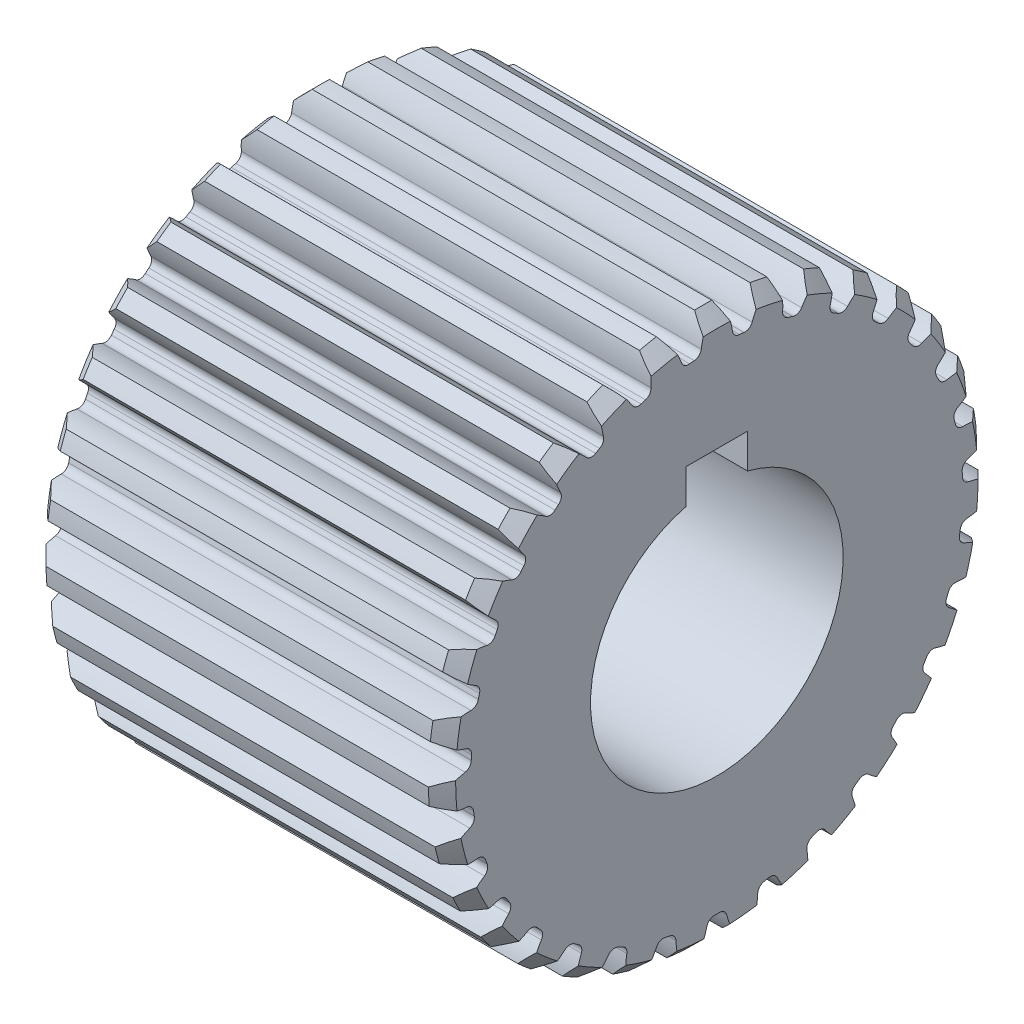
from build123d import *

# Parameters (mm, degrees)
SKETCH4_OUTSIDE_W   = 108.238
SKETCH4_OUTSIDE_H   = 108.238
CUT_EXTRUDE6_DEPTH  = 60
CUT_EXTRUDE7_REACH  = 84.701
SKETCH5_W           = 9
SKETCH5_H           = 23
BOSS_EXTRUDE1_DEPTH = 60
SCALE_1_SCALE       = 1.875


with BuildPart() as part:
    # Sketch1 → Revolve1 (revolve)
    with BuildSketch(Plane.XY, mode=Mode.PRIVATE) as revolve1_sk:
        Polygon((31.149526316, 18.25), (31.149526316, 38.25), (29.149526316, 40.25), (-26.850473684, 40.25), (-28.850473684, 38.25), (-28.850473684, 18.25), (-28.850473684, 0), (31.149526316, 0), align=None)
    revolve(revolve1_sk.sketch.rotate(Axis((-28.850473684, 0, 0), (1, 0, 0)), 90), axis=Axis((-28.850473684, 0, 0), (1, 0, 0)))

    # Sketch2 → Cut-Revolve1 (revolve, cut)
    with BuildSketch(Plane.XY, mode=Mode.PRIVATE) as cut_revolve1_sk:
        Polygon((0, 0), (44.149457516, 0), (44.149457516, 19), (-36.76595356, 19), (-36.76595356, 0), align=None)
    revolve(cut_revolve1_sk.sketch.rotate(Axis((-36.76595356, 0, 0), (1, 0, 0)), 90), axis=Axis((-36.76595356, 0, 0), (1, 0, 0)), mode=Mode.SUBTRACT)

    # Sketch4 outside → Cut-Extrude6 (cut)
    with BuildSketch(Plane.ZY.offset(28.850473684)):
        Rectangle(SKETCH4_OUTSIDE_W, SKETCH4_OUTSIDE_H)
        with BuildLine():
            ThreePointArc((1.260367328, 40.230261921), (0, 40.25), (-1.260367328, 40.230261921))
            ThreePointArc((-1.260367328, 40.230261921), (-1.890771319, 38.543683265), (-2.279945836, 36.785701483))
            ThreePointArc((-2.279945836, 36.785701483), (-2.625906951, 36.135179583), (-3.304440864, 35.84802185))
            ThreePointArc((-3.304440864, 35.84802185), (-3.642059592, 35.815295642), (-3.979354981, 35.779389793))
            ThreePointArc((-3.979354981, 35.779389793), (-4.701803692, 35.924081517), (-5.171632058, 36.491645735))
            ThreePointArc((-5.171632058, 36.491645735), (-5.906719281, 38.135301273), (-6.863724652, 39.660456174))
            ThreePointArc((-6.863724652, 39.660456174), (-8.102265434, 39.426080135), (-9.332859723, 39.153036018))
            ThreePointArc((-9.332859723, 39.153036018), (-9.61085352, 37.374082336), (-9.63818248, 35.573746289))
            ThreePointArc((-9.63818248, 35.573746289), (-9.846112655, 34.866899151), (-10.452952512, 34.449031681))
            ThreePointArc((-10.452952512, 34.449031681), (-10.777072427, 34.34901323), (-11.100235566, 34.245945313))
            ThreePointArc((-11.100235566, 34.245945313), (-11.837021939, 34.242247333), (-12.411482728, 34.703617723))
            ThreePointArc((-12.411482728, 34.703617723), (-13.462388099, 36.165655566), (-14.706814939, 37.466946691))
            ThreePointArc((-14.706814939, 37.466946691), (-15.872823168, 36.988051918), (-17.023263743, 36.47288022))
            ThreePointArc((-17.023263743, 36.47288022), (-16.937466247, 34.674382085), (-16.601830801, 32.905397744))
            ThreePointArc((-16.601830801, 32.905397744), (-16.663217349, 32.171163771), (-17.173519056, 31.639694108))
            ThreePointArc((-17.173519056, 31.639694108), (-17.470870651, 31.476478181), (-17.766671202, 31.310467809))
            ThreePointArc((-17.766671202, 31.310467809), (-18.487631117, 31.15853152), (-19.143205837, 31.494819525))
            ThreePointArc((-19.143205837, 31.494819525), (-20.466905167, 32.71538367), (-21.947806495, 33.739536009))
            ThreePointArc((-21.947806495, 33.739536009), (-22.993545658, 33.035728509), (-24.016733346, 32.299520421))
            ThreePointArc((-24.016733346, 32.299520421), (-23.570657117, 30.555108557), (-22.885798217, 28.889898348))
            ThreePointArc((-22.885798217, 28.889898348), (-22.798127968, 28.158337166), (-23.190999712, 27.53502374))
            ThreePointArc((-23.190999712, 27.53502374), (-23.449409378, 27.315292417), (-23.705737232, 27.093136073))
            ThreePointArc((-23.705737232, 27.093136073), (-24.381354505, 26.799181766), (-25.091203849, 26.996619714))
            ThreePointArc((-25.091203849, 26.996619714), (-26.633504733, 27.925740124), (-28.290252273, 28.630824758))
            ThreePointArc((-28.290252273, 28.630824758), (-29.172909686, 27.730918493), (-30.026955064, 26.80381446))
            ThreePointArc((-30.026955064, 26.80381446), (-29.238862515, 25.184905294), (-28.232818366, 23.691643119))
            ThreePointArc((-28.232818366, 23.691643119), (-27.999680549, 22.99270493), (-28.259038115, 22.303066265))
            ThreePointArc((-28.259038115, 22.303066265), (-28.46792653, 22.035815372), (-28.674287594, 21.766608164))
            ThreePointArc((-28.674287594, 21.766608164), (-29.276902375, 21.342670361), (-30.011965028, 21.39317512))
            ThreePointArc((-30.011965028, 21.39317512), (-31.709725486, 21.992813495), (-33.4744918, 22.349964178))
            ThreePointArc((-33.4744918, 22.349964178), (-34.157931364, 21.290801416), (-34.807869713, 20.210757186))
            ThreePointArc((-34.807869713, 20.210757186), (-33.710025446, 18.78362905), (-32.423983614, 17.523449238))
            ThreePointArc((-32.423983614, 17.523449238), (-32.054922918, 16.885748651), (-32.170148177, 16.158018637))
            ThreePointArc((-32.170148177, 16.158018637), (-32.320963425, 15.854189456), (-32.468909253, 15.548952759))
            ThreePointArc((-32.468909253, 15.548952759), (-32.973850422, 15.012387524), (-33.704032833, 14.913891424))
            ThreePointArc((-33.704032833, 14.913891424), (-35.487746352, 15.159498498), (-37.288281699, 15.154093438))
            ThreePointArc((-37.288281699, 15.154093438), (-37.744523319, 13.979036427), (-38.163746087, 12.790269139))
            ThreePointArc((-38.163746087, 12.790269139), (-36.801095974, 11.613348826), (-35.287707163, 10.637843285))
            ThreePointArc((-35.287707163, 10.637843285), (-34.797832977, 10.08748784), (-34.764208593, 9.351459827))
            ThreePointArc((-34.764208593, 9.351459827), (-34.850776279, 9.023491161), (-34.934249953, 8.694721401))
            ThreePointArc((-34.934249953, 8.694721401), (-35.320845158, 8.067495778), (-36.016253573, 7.82403126))
            ThreePointArc((-36.016253573, 7.82403126), (-37.812894712, 7.705551852), (-39.575484965, 7.337812332))
            ThreePointArc((-39.575484965, 7.337812332), (-39.785850054, 6.094968045), (-39.957194211, 4.84614597))
            ThreePointArc((-39.957194211, 4.84614597), (-38.385525309, 3.967616736), (-36.706747835, 3.316722779))
            ThreePointArc((-36.706747835, 3.316722779), (-36.116115665, 2.87624409), (-35.935018225, 2.162051153))
            ThreePointArc((-35.935018225, 2.162051153), (-35.953794258, 1.823370078), (-35.969378355, 1.484527127))
            ThreePointArc((-35.969378355, 1.484527127), (-36.221800344, 0.792319807), (-36.85396466, 0.413854337))
            ThreePointArc((-36.85396466, 0.413854337), (-38.58997872, -0.063860993), (-40.242463226, -0.778879672))
            ThreePointArc((-40.242463226, -0.778879672), (-40.198339414, -2.038629046), (-40.11479011, -3.296378984))
            ThreePointArc((-40.11479011, -3.296378984), (-38.398446728, -3.840550049), (-36.623009937, -4.140184747))
            ThreePointArc((-36.623009937, -4.140184747), (-35.955800335, -4.45275343), (-35.634643988, -5.115872149))
            ThreePointArc((-35.634643988, -5.115872149), (-35.584859676, -5.45139999), (-35.53191618, -5.786443862))
            ThreePointArc((-35.53191618, -5.786443862), (-35.639830767, -6.515293831), (-36.182870104, -7.013265831))
            ThreePointArc((-36.182870104, -7.013265831), (-37.787184465, -7.830659362), (-39.261910314, -8.863684252))
            ThreePointArc((-39.261910314, -8.863684252), (-38.965104034, -10.088764423), (-38.630081789, -11.303949796))
            ThreePointArc((-38.630081789, -11.303949796), (-36.839331227, -11.491484264), (-35.03992171, -11.427592624))
            ThreePointArc((-35.03992171, -11.427592624), (-34.323450314, -11.599454702), (-33.87538324, -12.184351044))
            ThreePointArc((-33.87538324, -12.184351044), (-33.759076757, -12.502989102), (-33.639773183, -12.820517159))
            ThreePointArc((-33.639773183, -12.820517159), (-33.598762332, -13.556170573), (-34.030444595, -14.153262072))
            ThreePointArc((-34.030444595, -14.153262072), (-35.437378438, -15.276869616), (-36.673970181, -16.585608556))
            ThreePointArc((-36.673970181, -16.585608556), (-36.136632718, -17.7258646), (-35.56385338, -18.848735574))
            ThreePointArc((-35.56385338, -18.848735574), (-33.772009176, -18.671955763), (-32.02229497, -18.247153516))
            ThreePointArc((-32.02229497, -18.247153516), (-31.285894204, -18.271272935), (-30.729260321, -18.754001176))
            ThreePointArc((-30.729260321, -18.754001176), (-30.55119327, -19.042704372), (-30.370413918, -19.329716977))
            ThreePointArc((-30.370413918, -19.329716977), (-30.182156618, -20.042056099), (-30.484808685, -20.713822101))
            ThreePointArc((-30.484808685, -20.713822101), (-31.636761975, -22.097643033), (-32.584593399, -23.628516098))
            ThreePointArc((-32.584593399, -23.628516098), (-31.828723412, -24.637265798), (-31.041636636, -25.621851904))
            ThreePointArc((-31.041636636, -25.621851904), (-29.322057102, -25.0879952), (-27.693671712, -24.319673799))
            ThreePointArc((-27.693671712, -24.319673799), (-26.96748991, -24.195063108), (-26.325077874, -24.555860297))
            ThreePointArc((-26.325077874, -24.555860297), (-26.09254034, -24.802809087), (-25.85768634, -25.047555912))
            ThreePointArc((-25.85768634, -25.047555912), (-25.529889867, -25.707417493), (-25.691121126, -26.426355819))
            ThreePointArc((-25.691121126, -26.426355819), (-26.540932759, -28.013736347), (-27.161199536, -29.704069414))
            ThreePointArc((-27.161199536, -29.704069414), (-26.21774243, -30.540014438), (-25.24857164, -31.346006606))
            ThreePointArc((-25.24857164, -31.346006606), (-23.671656565, -30.476929165), (-22.231266281, -29.396543779))
            ThreePointArc((-22.231266281, -29.396543779), (-21.54503341, -29.128304554), (-20.843143647, -29.352399611))
            ThreePointArc((-20.843143647, -29.352399611), (-20.565655743, -29.547483883), (-20.286342045, -29.739944964))
            ThreePointArc((-20.286342045, -29.739944964), (-19.832426425, -30.320314195), (-19.84563605, -31.056991425))
            ThreePointArc((-19.84563605, -31.056991425), (-20.358514637, -32.782944005), (-20.625822972, -34.563534639))
            ThreePointArc((-20.625822972, -34.563534639), (-19.533403992, -35.1924513), (-18.421827155, -35.786852115))
            ThreePointArc((-18.421827155, -35.786852115), (-17.052135627, -34.618134069), (-15.858710196, -33.269915803))
            ThreePointArc((-15.858710196, -33.269915803), (-15.240520711, -32.869029789), (-14.507888669, -32.947248237))
            ThreePointArc((-14.507888669, -32.947248237), (-14.196810784, -33.082481218), (-13.884472522, -33.214777175))
            ThreePointArc((-13.884472522, -33.214777175), (-13.323021115, -33.691893672), (-13.187668302, -34.416150153))
            ThreePointArc((-13.187668302, -34.416150153), (-13.342616534, -36.210014083), (-13.246022792, -38.007964694))
            ThreePointArc((-13.246022792, -38.007964694), (-12.0493657, -38.40410507), (-10.840890901, -38.762579693))
            ThreePointArc((-10.840890901, -38.762579693), (-9.734498252, -37.342068497), (-8.836896652, -35.781213565))
            ThreePointArc((-8.836896652, -35.781213565), (-8.312059304, -35.264093083), (-7.578679025, -35.193232648))
            ThreePointArc((-7.578679025, -35.193232648), (-7.246746723, -35.263077885), (-6.914171064, -35.329792506))
            ThreePointArc((-6.914171064, -35.329792506), (-6.268169755, -35.684123062), (-5.989795864, -36.36630765))
            ThreePointArc((-5.989795864, -36.36630765), (-5.780470142, -38.154641929), (-5.323928883, -39.896344209))
            ThreePointArc((-5.323928883, -39.896344209), (-4.07202496, -40.043490267), (-2.8161273, -40.151362704))
            ThreePointArc((-2.8161273, -40.151362704), (-2.018329376, -38.537214253), (-1.453299521, -36.827624239))
            ThreePointArc((-1.453299521, -36.827624239), (-1.043301211, -36.215440262), (-0.33919737, -35.99840198))
            ThreePointArc((-0.33919737, -35.99840198), (0, -36), (0.33919737, -35.99840198))
            ThreePointArc((0.33919737, -35.99840198), (1.043301211, -36.215440262), (1.453299521, -36.827624239))
            ThreePointArc((1.453299521, -36.827624239), (2.018329376, -38.537214253), (2.8161273, -40.151362704))
            ThreePointArc((2.8161273, -40.151362704), (4.07202496, -40.043490267), (5.323928883, -39.896344209))
            ThreePointArc((5.323928883, -39.896344209), (5.780470142, -38.154641929), (5.989795864, -36.36630765))
            ThreePointArc((5.989795864, -36.36630765), (6.268169755, -35.684123062), (6.914171064, -35.329792506))
            ThreePointArc((6.914171064, -35.329792506), (7.246746723, -35.263077885), (7.578679025, -35.193232648))
            ThreePointArc((7.578679025, -35.193232648), (8.312059304, -35.264093083), (8.836896652, -35.781213565))
            ThreePointArc((8.836896652, -35.781213565), (9.734498252, -37.342068497), (10.840890901, -38.762579693))
            ThreePointArc((10.840890901, -38.762579693), (12.0493657, -38.40410507), (13.246022792, -38.007964694))
            ThreePointArc((13.246022792, -38.007964694), (13.342616534, -36.210014083), (13.187668302, -34.416150153))
            ThreePointArc((13.187668302, -34.416150153), (13.323021115, -33.691893672), (13.884472522, -33.214777175))
            ThreePointArc((13.884472522, -33.214777175), (14.196810784, -33.082481218), (14.507888669, -32.947248237))
            ThreePointArc((14.507888669, -32.947248237), (15.240520711, -32.869029789), (15.858710196, -33.269915803))
            ThreePointArc((15.858710196, -33.269915803), (17.052135627, -34.618134069), (18.421827155, -35.786852115))
            ThreePointArc((18.421827155, -35.786852115), (19.533403992, -35.1924513), (20.625822972, -34.563534639))
            ThreePointArc((20.625822972, -34.563534639), (20.358514637, -32.782944005), (19.84563605, -31.056991425))
            ThreePointArc((19.84563605, -31.056991425), (19.832426425, -30.320314195), (20.286342045, -29.739944964))
            ThreePointArc((20.286342045, -29.739944964), (20.565655743, -29.547483883), (20.843143647, -29.352399611))
            ThreePointArc((20.843143647, -29.352399611), (21.54503341, -29.128304554), (22.231266281, -29.396543779))
            ThreePointArc((22.231266281, -29.396543779), (23.671656565, -30.476929165), (25.24857164, -31.346006606))
            ThreePointArc((25.24857164, -31.346006606), (26.21774243, -30.540014438), (27.161199536, -29.704069414))
            ThreePointArc((27.161199536, -29.704069414), (26.540932759, -28.013736347), (25.691121126, -26.426355819))
            ThreePointArc((25.691121126, -26.426355819), (25.529889867, -25.707417493), (25.85768634, -25.047555912))
            ThreePointArc((25.85768634, -25.047555912), (26.09254034, -24.802809087), (26.325077874, -24.555860297))
            ThreePointArc((26.325077874, -24.555860297), (26.96748991, -24.195063108), (27.693671712, -24.319673799))
            ThreePointArc((27.693671712, -24.319673799), (29.322057102, -25.0879952), (31.041636636, -25.621851904))
            ThreePointArc((31.041636636, -25.621851904), (31.828723412, -24.637265798), (32.584593399, -23.628516098))
            ThreePointArc((32.584593399, -23.628516098), (31.636761975, -22.097643033), (30.484808685, -20.713822101))
            ThreePointArc((30.484808685, -20.713822101), (30.182156618, -20.042056099), (30.370413918, -19.329716977))
            ThreePointArc((30.370413918, -19.329716977), (30.55119327, -19.042704372), (30.729260321, -18.754001176))
            ThreePointArc((30.729260321, -18.754001176), (31.285894204, -18.271272935), (32.02229497, -18.247153516))
            ThreePointArc((32.02229497, -18.247153516), (33.772009176, -18.671955763), (35.56385338, -18.848735574))
            ThreePointArc((35.56385338, -18.848735574), (36.136632718, -17.7258646), (36.673970181, -16.585608556))
            ThreePointArc((36.673970181, -16.585608556), (35.437378438, -15.276869616), (34.030444595, -14.153262072))
            ThreePointArc((34.030444595, -14.153262072), (33.598762332, -13.556170573), (33.639773183, -12.820517159))
            ThreePointArc((33.639773183, -12.820517159), (33.759076757, -12.502989102), (33.87538324, -12.184351044))
            ThreePointArc((33.87538324, -12.184351044), (34.323450314, -11.599454702), (35.03992171, -11.427592624))
            ThreePointArc((35.03992171, -11.427592624), (36.839331227, -11.491484264), (38.630081789, -11.303949796))
            ThreePointArc((38.630081789, -11.303949796), (38.965104034, -10.088764423), (39.261910314, -8.863684252))
            ThreePointArc((39.261910314, -8.863684252), (37.787184465, -7.830659362), (36.182870104, -7.013265831))
            ThreePointArc((36.182870104, -7.013265831), (35.639830767, -6.515293831), (35.53191618, -5.786443862))
            ThreePointArc((35.53191618, -5.786443862), (35.584859676, -5.45139999), (35.634643988, -5.115872149))
            ThreePointArc((35.634643988, -5.115872149), (35.955800335, -4.45275343), (36.623009937, -4.140184747))
            ThreePointArc((36.623009937, -4.140184747), (38.398446728, -3.840550049), (40.11479011, -3.296378984))
            ThreePointArc((40.11479011, -3.296378984), (40.198339414, -2.038629046), (40.242463226, -0.778879672))
            ThreePointArc((40.242463226, -0.778879672), (38.58997872, -0.063860993), (36.85396466, 0.413854337))
            ThreePointArc((36.85396466, 0.413854337), (36.221800344, 0.792319807), (35.969378355, 1.484527127))
            ThreePointArc((35.969378355, 1.484527127), (35.953794258, 1.823370078), (35.935018225, 2.162051153))
            ThreePointArc((35.935018225, 2.162051153), (36.116115665, 2.87624409), (36.706747835, 3.316722779))
            ThreePointArc((36.706747835, 3.316722779), (38.385525309, 3.967616736), (39.957194211, 4.84614597))
            ThreePointArc((39.957194211, 4.84614597), (39.785850054, 6.094968045), (39.575484965, 7.337812332))
            ThreePointArc((39.575484965, 7.337812332), (37.812894712, 7.705551852), (36.016253573, 7.82403126))
            ThreePointArc((36.016253573, 7.82403126), (35.320845158, 8.067495778), (34.934249953, 8.694721401))
            ThreePointArc((34.934249953, 8.694721401), (34.850776279, 9.023491161), (34.764208593, 9.351459827))
            ThreePointArc((34.764208593, 9.351459827), (34.797832977, 10.08748784), (35.287707163, 10.637843285))
            ThreePointArc((35.287707163, 10.637843285), (36.801095974, 11.613348826), (38.163746087, 12.790269139))
            ThreePointArc((38.163746087, 12.790269139), (37.744523319, 13.979036427), (37.288281699, 15.154093438))
            ThreePointArc((37.288281699, 15.154093438), (35.487746352, 15.159498498), (33.704032833, 14.913891424))
            ThreePointArc((33.704032833, 14.913891424), (32.973850422, 15.012387524), (32.468909253, 15.548952759))
            ThreePointArc((32.468909253, 15.548952759), (32.320963425, 15.854189456), (32.170148177, 16.158018637))
            ThreePointArc((32.170148177, 16.158018637), (32.054922918, 16.885748651), (32.423983614, 17.523449238))
            ThreePointArc((32.423983614, 17.523449238), (33.710025446, 18.78362905), (34.807869713, 20.210757186))
            ThreePointArc((34.807869713, 20.210757186), (34.157931364, 21.290801416), (33.4744918, 22.349964178))
            ThreePointArc((33.4744918, 22.349964178), (31.709725486, 21.992813495), (30.011965028, 21.39317512))
            ThreePointArc((30.011965028, 21.39317512), (29.276902375, 21.342670361), (28.674287594, 21.766608164))
            ThreePointArc((28.674287594, 21.766608164), (28.46792653, 22.035815372), (28.259038115, 22.303066265))
            ThreePointArc((28.259038115, 22.303066265), (27.999680549, 22.99270493), (28.232818366, 23.691643119))
            ThreePointArc((28.232818366, 23.691643119), (29.238862515, 25.184905294), (30.026955064, 26.80381446))
            ThreePointArc((30.026955064, 26.80381446), (29.172909686, 27.730918493), (28.290252273, 28.630824758))
            ThreePointArc((28.290252273, 28.630824758), (26.633504733, 27.925740124), (25.091203849, 26.996619714))
            ThreePointArc((25.091203849, 26.996619714), (24.381354505, 26.799181766), (23.705737232, 27.093136073))
            ThreePointArc((23.705737232, 27.093136073), (23.449409378, 27.315292417), (23.190999712, 27.53502374))
            ThreePointArc((23.190999712, 27.53502374), (22.798127968, 28.158337166), (22.885798217, 28.889898348))
            ThreePointArc((22.885798217, 28.889898348), (23.570657117, 30.555108557), (24.016733346, 32.299520421))
            ThreePointArc((24.016733346, 32.299520421), (22.993545658, 33.035728509), (21.947806495, 33.739536009))
            ThreePointArc((21.947806495, 33.739536009), (20.466905167, 32.71538367), (19.143205837, 31.494819525))
            ThreePointArc((19.143205837, 31.494819525), (18.487631117, 31.15853152), (17.766671202, 31.310467809))
            ThreePointArc((17.766671202, 31.310467809), (17.470870651, 31.476478181), (17.173519056, 31.639694108))
            ThreePointArc((17.173519056, 31.639694108), (16.663217349, 32.171163771), (16.601830801, 32.905397744))
            ThreePointArc((16.601830801, 32.905397744), (16.937466247, 34.674382085), (17.023263743, 36.47288022))
            ThreePointArc((17.023263743, 36.47288022), (15.872823168, 36.988051918), (14.706814939, 37.466946691))
            ThreePointArc((14.706814939, 37.466946691), (13.462388099, 36.165655566), (12.411482728, 34.703617723))
            ThreePointArc((12.411482728, 34.703617723), (11.837021939, 34.242247333), (11.100235566, 34.245945313))
            ThreePointArc((11.100235566, 34.245945313), (10.777072427, 34.34901323), (10.452952512, 34.449031681))
            ThreePointArc((10.452952512, 34.449031681), (9.846112655, 34.866899151), (9.63818248, 35.573746289))
            ThreePointArc((9.63818248, 35.573746289), (9.61085352, 37.374082336), (9.332859723, 39.153036018))
            ThreePointArc((9.332859723, 39.153036018), (8.102265434, 39.426080135), (6.863724652, 39.660456174))
            ThreePointArc((6.863724652, 39.660456174), (5.906719281, 38.135301273), (5.171632058, 36.491645735))
            ThreePointArc((5.171632058, 36.491645735), (4.701803692, 35.924081517), (3.979354981, 35.779389793))
            ThreePointArc((3.979354981, 35.779389793), (3.642059592, 35.815295642), (3.304440864, 35.84802185))
            ThreePointArc((3.304440864, 35.84802185), (2.625906951, 36.135179583), (2.279945836, 36.785701483))
            ThreePointArc((2.279945836, 36.785701483), (1.890771319, 38.543683265), (1.260367328, 40.230261921))
        make_face(mode=Mode.SUBTRACT)
    extrude(amount=-CUT_EXTRUDE6_DEPTH, mode=Mode.SUBTRACT)

    # Sketch5 → Cut-Extrude7 (cut, up to next)
    with BuildSketch(Plane.ZY.offset(28.850473684), mode=Mode.PRIVATE) as cut_extrude7_sk1:
        with Locations((0, 11.5)):
            Rectangle(SKETCH5_W, SKETCH5_H)
    cut_extrude7_tool1 = extrude(cut_extrude7_sk1.sketch, amount=-CUT_EXTRUDE7_REACH, mode=Mode.PRIVATE) & part.part
    add(cut_extrude7_tool1.solids().sort_by_distance((-28.850474, 11.5, 0))[0], mode=Mode.SUBTRACT)

    # Sketch7 → Boss-Extrude1 (add)
    with BuildSketch(Plane.ZY.offset(28.850473684)):
        with BuildLine():
            Line((4.5, 18.459414942), (4.5, 17.944358445))
            ThreePointArc((4.5, 17.944358445), (0, -18.5), (-4.5, 17.944358445))
            Line((-4.5, 17.944358445), (-4.5, 18.459414942))
            ThreePointArc((-4.5, 18.459414942), (0, -19), (4.5, 18.459414942))
        make_face()
    extrude(amount=-BOSS_EXTRUDE1_DEPTH)


with BuildPart() as part_1:
    # Scale 1: scaled about (1.149526316, -0.25074678, 0)
    add(part.part.scale(SCALE_1_SCALE).moved(Location((-1.005835527, 0.219403432, 0))))


solid = part_1.part
